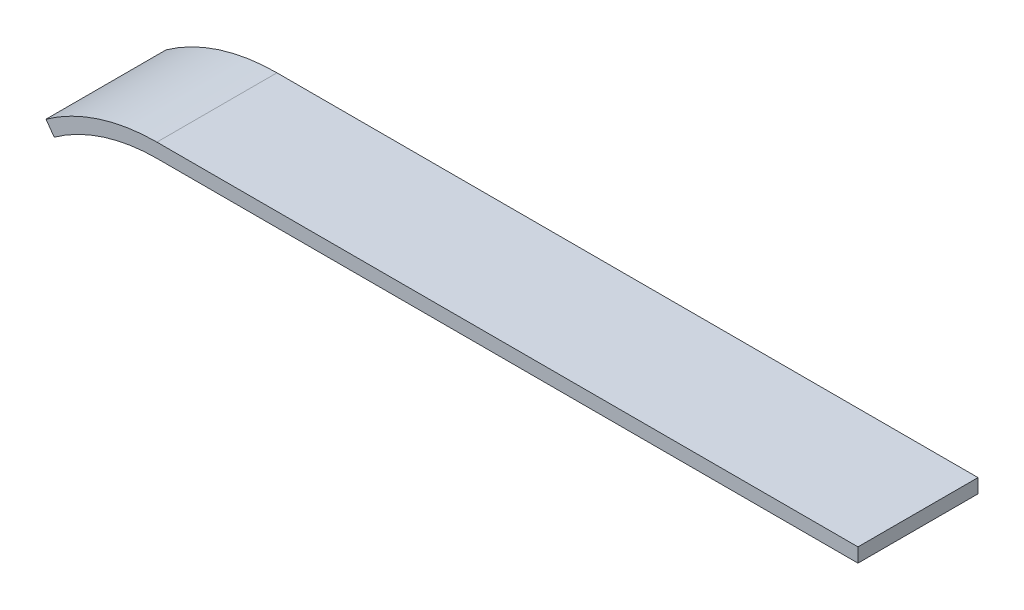
from build123d import *

# Parameters (mm, degrees)
BOSS_EXTRUDE1_DEPTH = 102


with BuildPart() as part:
    # Sketch1 → Boss-Extrude1 (new body)
    with BuildSketch(Plane.XY):
        with BuildLine():
            Line((0, 0), (-595.74872733, 0))
            ThreePointArc((-595.74872733, 0), (-645.240544835, -7.745145943), (-690, -30.24))
            Line((-690, -30.24), (-683.018424247, -40))
            ThreePointArc((-683.018424247, -40), (-641.574484279, -19.171431429), (-595.74872733, -12))
            Line((-595.74872733, -12), (0, -12))
            Line((0, -12), (0, 0))
        make_face()
    extrude(amount=BOSS_EXTRUDE1_DEPTH)


solid = part.part
